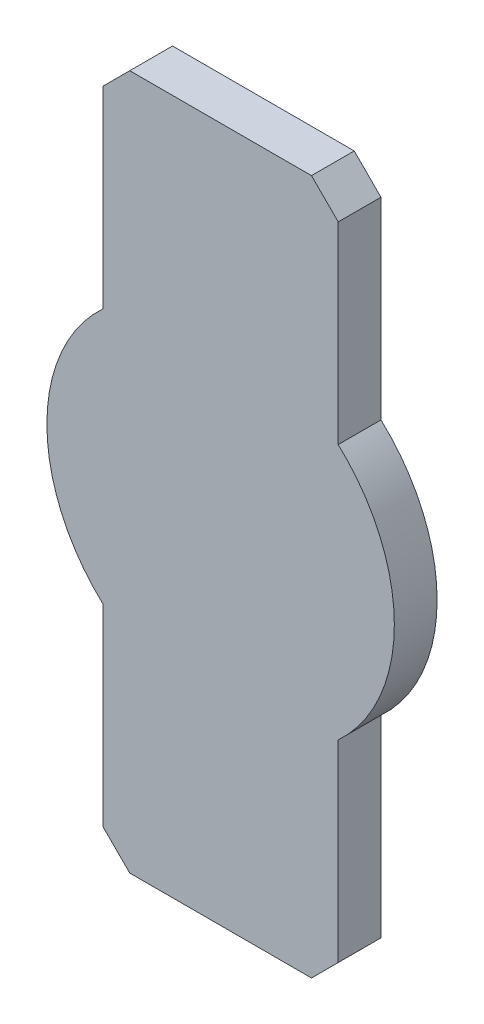
SolidWorks part; units mm, degrees
ref_plane "前视基准面" through (0, 0, 0) normal (0, 0, 1) x (1, 0, 0)
ref_plane "上视基准面" through (0, 0, 0) normal (0, 1, 0) x (1, 0, 0)
ref_plane "右视基准面" through (0, 0, 0) normal (1, 0, 0) x (0, 0, -1)
sketch "草图1" plane through (0, 0, 0) normal (0, 0, 1) x (1, 0, 0)
  circle A0 centre (0, 0) radius 32.5
  dimension "D1" = 65
extrude "凸台-拉伸1" add sketch "草图1" along normal mid plane 8
sketch "草图2" plane through (0, 0, 4) normal (0, 0, 1) x (1, 0, 0)
  line L1 (-22, 65) -> (22, 65)
  line L2 (-22, 65) -> (-22, -65)
  line L3 (-22, -65) -> (22, -65)
  line L4 (22, 65) -> (22, -65)
  line L5 (-22, 65) -> (22, -65) construction
  line L6 (-22, -65) -> (22, 65) construction
  point P0 (0, 0)
  dimension "D1" = 44
  dimension "D2" = 130
extrude "凸台-拉伸2" add sketch "草图2" against normal up to surface (8 mm away) up to face at (32.5, 0, -4)
chamfer "倒角1" distance 5 angle 45 4 edges at (22, -65, 0) (22, 65, 0) (-22, -65, 0) (-22, 65, 0)
